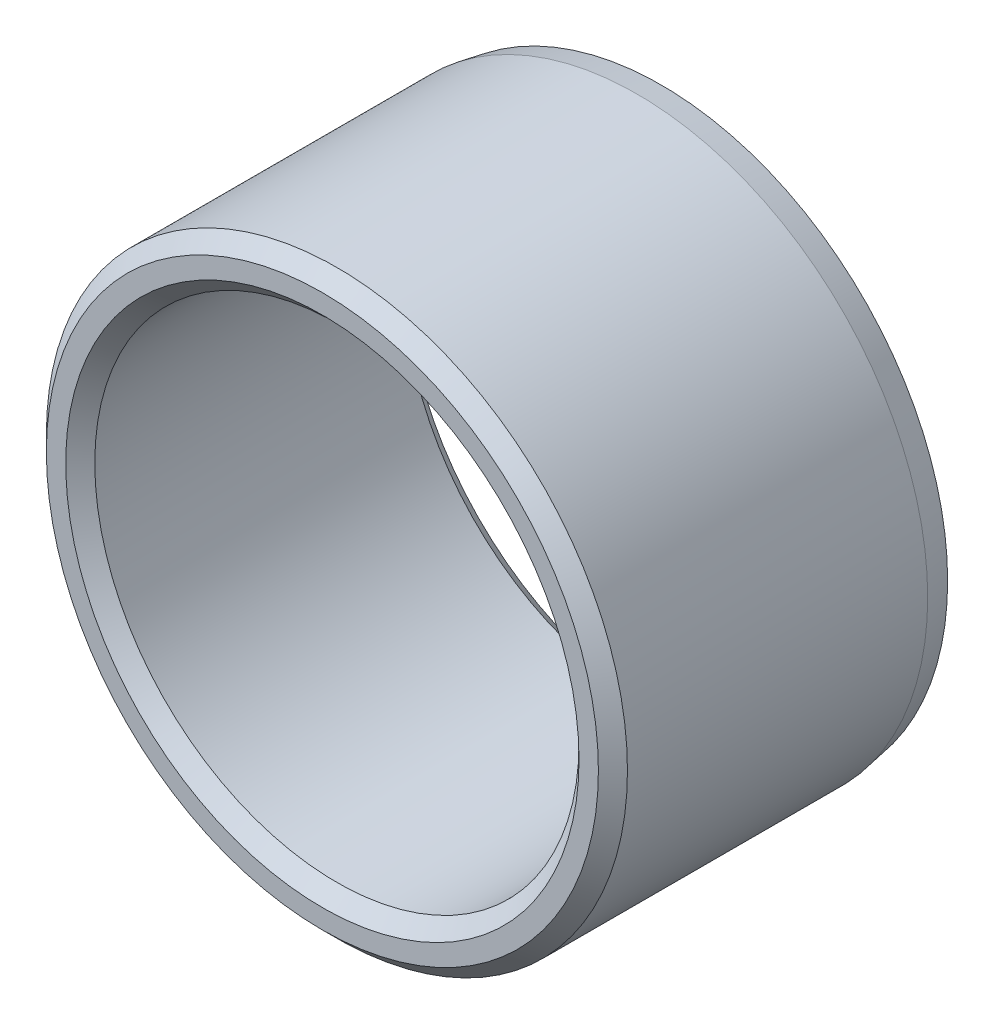
SolidWorks part; units mm, degrees
material "ZCuSn3Zn8Pb6Ni1"
ref_plane "Front Plane" through (0, 0, 0) normal (0, 0, 1) x (1, 0, 0)
ref_plane "Top Plane" through (0, 0, 0) normal (0, 1, 0) x (1, 0, 0)
ref_plane "Right Plane" through (0, 0, 0) normal (1, 0, 0) x (0, 0, -1)
sketch "Sketch1" plane through (0, 0, 0) normal (0, 0, 1) x (1, 0, 0)
  circle A0 centre (0, 0) radius 50
  circle A1 centre (0, 0) radius 60
  dimension "D1" = 100
  dimension "D2" = 120
extrude "Boss-Extrude1" add sketch "Sketch1" along normal mid plane 70
chamfer "Chamfer1" distance 3 angle 45 3 edges at (50, 0, -35) (50, 0, 35) (60, 0, 35)
chamfer "Chamfer2" distance 5 angle 10 1 edges at (60, 0, -35)
